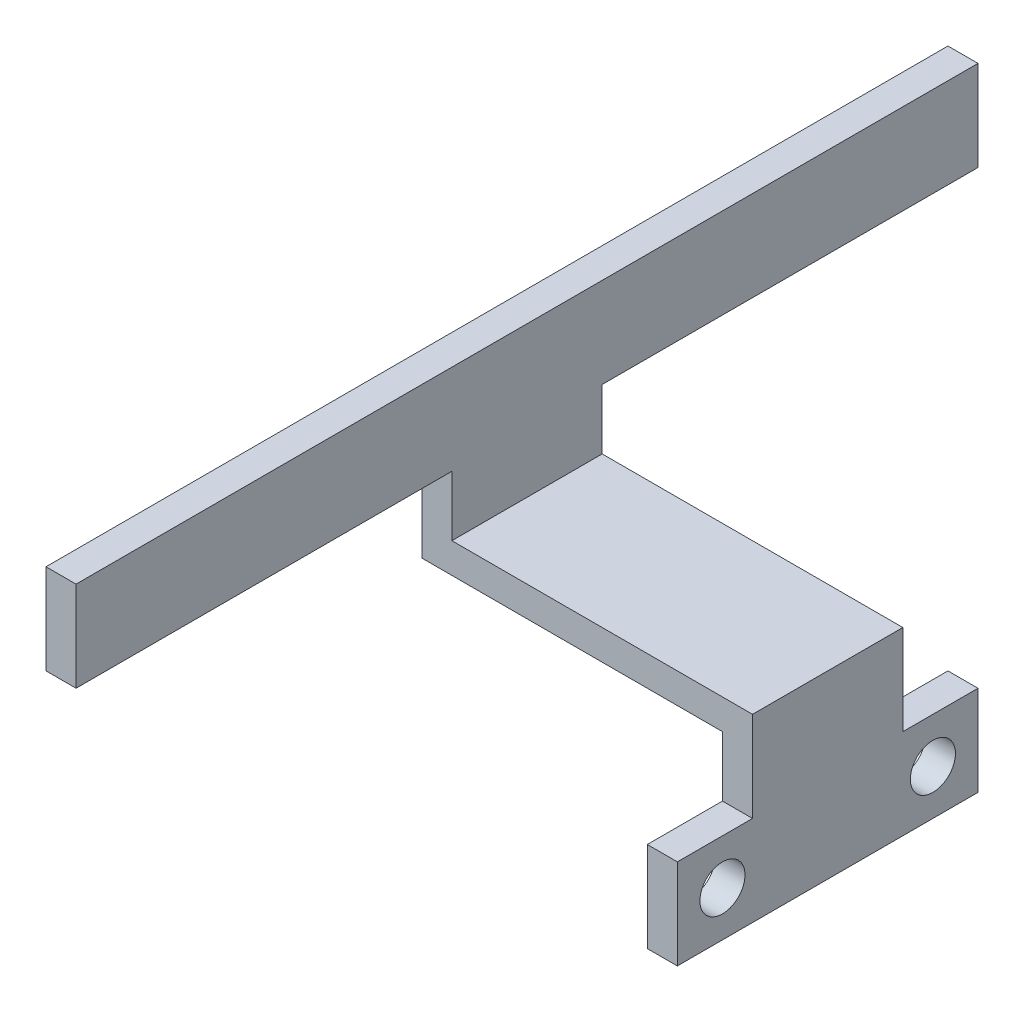
from build123d import *

# Parameters (mm, degrees)
BOSS_EXTRUDE1_DEPTH = 5
SKETCH2_W           = 20
SKETCH2_H           = 6
SKETCH2_R           = 1.5
BOSS_EXTRUDE2_DEPTH = 2
SKETCH3_W           = 60
SKETCH3_H           = 6
BOSS_EXTRUDE3_DEPTH = 2


with BuildPart() as part:
    # Sketch1 → Boss-Extrude1 (new, symmetric)
    with BuildSketch(Plane.XY):
        Polygon((-14.216216216, 5.673798061), (-14.216216216, 15.673798061), (-16.216216216, 15.673798061), (-16.216216216, 3.673798061), (3.783783784, 3.673798061), (3.783783784, -6.326201939), (5.783783784, -6.326201939), (5.783783784, 5.673798061), align=None)
    extrude(amount=BOSS_EXTRUDE1_DEPTH, both=True)

    # Sketch2 → Boss-Extrude2 (add)
    with BuildSketch(Plane(origin=(5.783783784, 0, 0), x_dir=(0, 0, -1), z_dir=(1, 0, 0))):
        with Locations((0, -3.326201939)):
            Rectangle(SKETCH2_W, SKETCH2_H)
        with Locations((-7, -3.326201939)):
            Circle(SKETCH2_R, mode=Mode.SUBTRACT)
        with Locations((7, -3.326201939)):
            Circle(SKETCH2_R, mode=Mode.SUBTRACT)
    extrude(amount=-BOSS_EXTRUDE2_DEPTH)

    # Sketch3 → Boss-Extrude3 (add)
    with BuildSketch(Plane.ZY.offset(16.216216216)):
        with Locations((0, 12.673798061)):
            Rectangle(SKETCH3_W, SKETCH3_H)
    extrude(amount=-BOSS_EXTRUDE3_DEPTH)


solid = part.part
